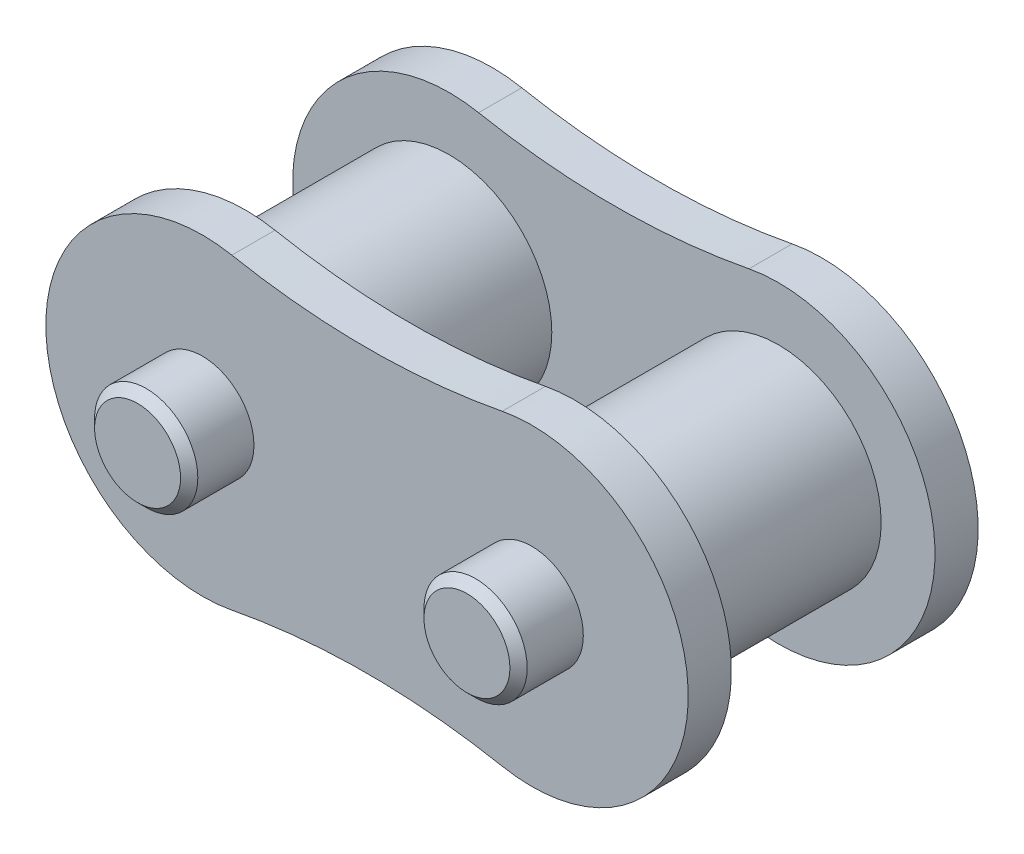
from build123d import *

# Parameters (mm, degrees)
SKETCH_2_R                 = 3.96
EXTRUDE_1_DEPTH            = 3.925
EXTRUDE_1_2_DEPTH          = 3.925
EXTRUDE_2_DEPTH            = 1.665
SKETCH_4_R                 = 1.99
EXTRUDE_3_DEPTH            = 2.4975
CHAMFER_1_SIZE             = 0.333
CHAMFER_1_OF_MIRROR_1_SIZE = 0.333


with BuildPart() as part:
    # 草图2 → 拉伸1 (new, symmetric)
    with BuildSketch(Plane.XY):
        with Locations((6.35, 0)):
            Circle(SKETCH_2_R)
    extrude(amount=EXTRUDE_1_DEPTH, both=True)



with BuildPart() as body_2:
    # 草图2 → Extrude 1 2 (new, symmetric)
    with BuildSketch(Plane.XY):
        with Locations((-6.35, 0)):
            Circle(SKETCH_2_R)
    extrude(amount=EXTRUDE_1_2_DEPTH, both=True)


with BuildPart() as part_1:
    add(part.part)

    add(body_2.part)  # 拉伸2 merges body 2
    # 草图3 → 拉伸2 (add)
    with BuildSketch(Plane.XY.offset(3.925)):
        with BuildLine():
            ThreePointArc((-5.213143439, 5.926953869), (-12.385, 0), (-5.213143439, -5.926953869))
            ThreePointArc((-5.213143439, -5.926953869), (0, -5.4315), (5.213143439, -5.926953869))
            ThreePointArc((5.213143439, -5.926953869), (12.385, 0), (5.213143439, 5.926953869))
            ThreePointArc((5.213143439, 5.926953869), (0, 5.4315), (-5.213143439, 5.926953869))
        make_face()
    extrude_2 = extrude(amount=EXTRUDE_2_DEPTH)

    # 草图4 → 拉伸3 (add)
    with BuildSketch(Plane.XY.offset(5.59)):
        with Locations((6.35, 0)):
            Circle(SKETCH_4_R)
        with Locations((-6.35, 0)):
            Circle(SKETCH_4_R)
    extrude_3 = extrude(amount=EXTRUDE_3_DEPTH)

    # 倒角1
    chamfer_1_edges = [part_1.edges().sort_by_distance(p)[0] for p in [
        (4.36, 0, 8.0875),
        (-8.34, 0, 8.0875),
    ]]
    chamfer(chamfer_1_edges, length=CHAMFER_1_SIZE)

    # 镜向1: 拉伸2, 拉伸3 across plane
    add(extrude_2.mirror(Plane.XY))
    add(extrude_3.mirror(Plane.XY))

    # 倒角1 of 镜向1
    chamfer_1_of_mirror_1_edges = [part_1.edges().sort_by_distance(p)[0] for p in [
        (4.36, 0, -8.0875),
        (-8.34, 0, -8.0875),
    ]]
    chamfer(chamfer_1_of_mirror_1_edges, length=CHAMFER_1_OF_MIRROR_1_SIZE)


solid = part_1.part
